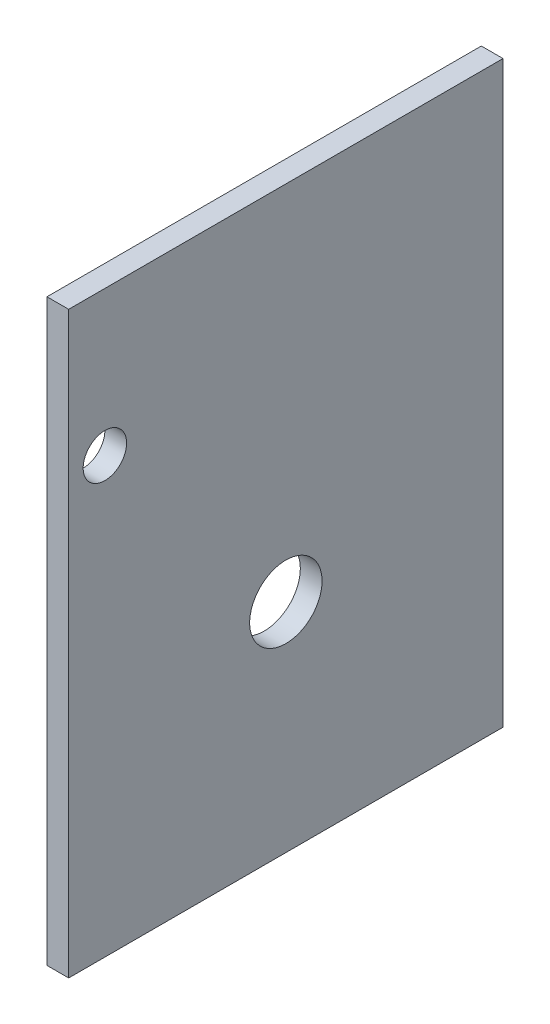
SolidWorks part; units mm, degrees
ref_plane "Front Plane" through (0, 0, 0) normal (0, 0, 1) x (1, 0, 0)
ref_plane "Top Plane" through (0, 0, 0) normal (0, 1, 0) x (1, 0, 0)
ref_plane "Right Plane" through (0, 0, 0) normal (1, 0, 0) x (0, 0, -1)
other "Configuration Table"
sketch "Sketch1" plane through (0, 0, 0) normal (1, 0, 0) x (0, 0, -1)
  line L1 (-30, -40) -> (30, -40)
  line L2 (-30, -40) -> (-30, 40)
  line L3 (-30, 40) -> (30, 40)
  line L4 (30, -40) -> (30, 40)
  line L5 (0, 40) -> (0, -40) construction
  line L6 (-30, 0) -> (30, 0) construction
  circle A0 centre (-25, 20) radius 3
  circle A1 centre (0, -10) radius 3
  point P0 (0, 0)
  dimension "D3" = 6
  dimension "D4" = 5
  dimension "D5" = 20
  dimension "D6" = 6
  dimension "D7" = 50
  dimension "D8" = 30
  dimension "D1" = 80
  dimension "D2" = 60
extrude "Boss-Extrude1" add sketch "Sketch1" along normal blind 3
sketch "Sketch2" plane through (3, 0, 0) normal (1, 0, 0) x (0, 0, -1)
  circle A0 centre (0, -10) radius 5
  dimension "D1" = 10
extrude "Cut-Extrude1" cut sketch "Sketch2" against normal blind 3
